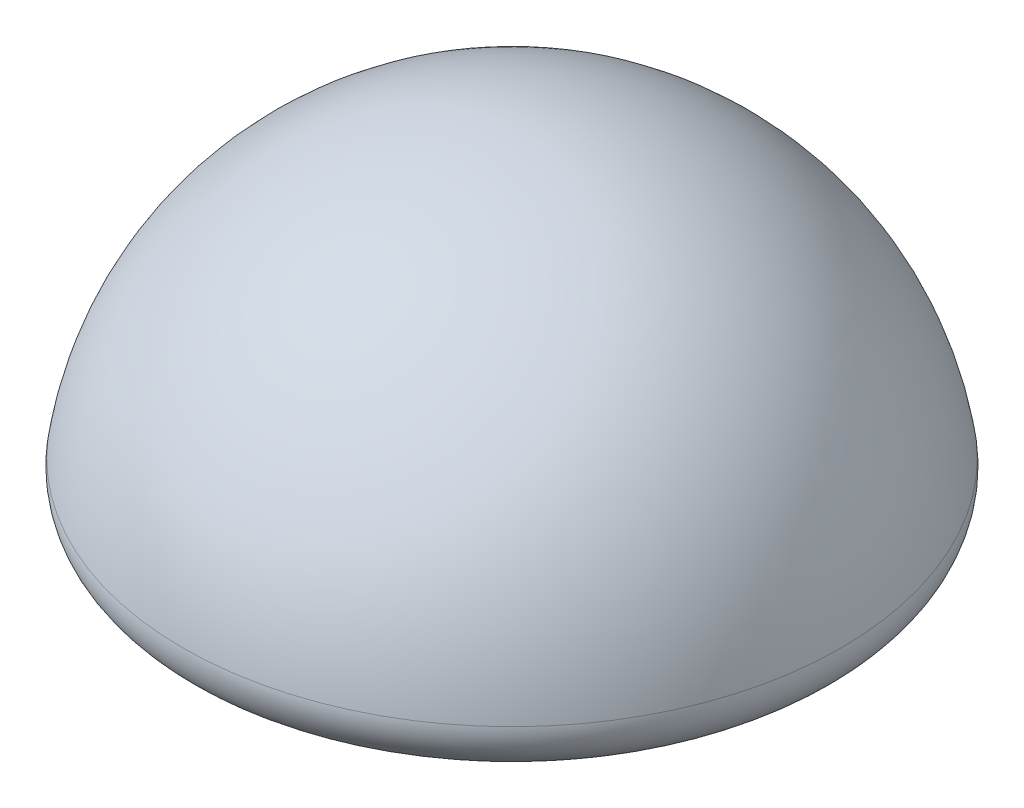
from build123d import *

# Parameters (mm, degrees)
SKETCH_2_R      = 5
EXTRUDE_1_DEPTH = 2
FILLET_1_R      = 2


with BuildPart() as part:
    # 草图1 → 旋转1 (revolve)
    with BuildSketch(Plane.XY):
        with BuildLine():
            Line((0, 15), (0, 0))
            Line((0, 0), (15, 0))
            ThreePointArc((15, 0), (10.606601718, 10.606601718), (0, 15))
        make_face()
    revolve(axis=Axis((0, 0, 0), (0, 1, 0)))

    # 草图2 → 凸台-拉伸1 (add)
    with BuildSketch(Plane.XZ):
        with Locations(Location((0, 0, 0), (0, 0, 270))):
            Circle(SKETCH_2_R)
    extrude(amount=EXTRUDE_1_DEPTH)

    # 圆角1
    fillet_1_edges = [part.edges().sort_by_distance(p)[0] for p in [
        (-15, 0, 0),
    ]]
    fillet(fillet_1_edges, radius=FILLET_1_R)


solid = part.part
